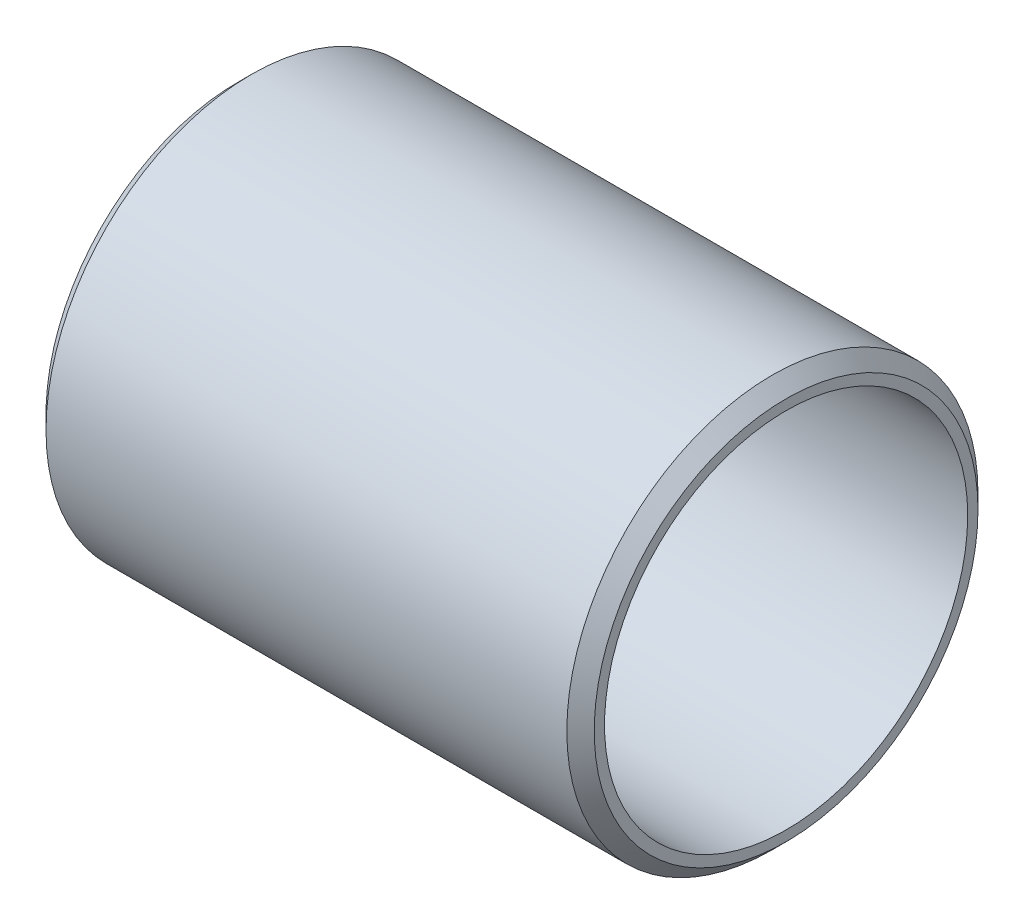
SolidWorks part; units mm, degrees
material "镀锌焊接钢管 Q215A"
ref_plane "前视基准面" through (0, 0, 0) normal (0, 0, 1) x (1, 0, 0)
ref_plane "上视基准面" through (0, 0, 0) normal (0, 1, 0) x (1, 0, 0)
ref_plane "右视基准面" through (0, 0, 0) normal (1, 0, 0) x (0, 0, -1)
sketch "草图1" plane through (0, 0, 0) normal (1, 0, 0) x (0, 0, -1)
  circle A0 centre (0, 0) radius 30
  dimension "D1" = 60
extrude "拉伸-薄壁1" add sketch "草图1" along normal blind 80 thin thin type one direction reverse wall 3.5
cosmetic thread "装饰螺纹线1"
cosmetic thread "装饰螺纹线2"
chamfer "倒角1" distance 2 angle 45 2 edges at (80, 0, -30) (0, 0, -30)
